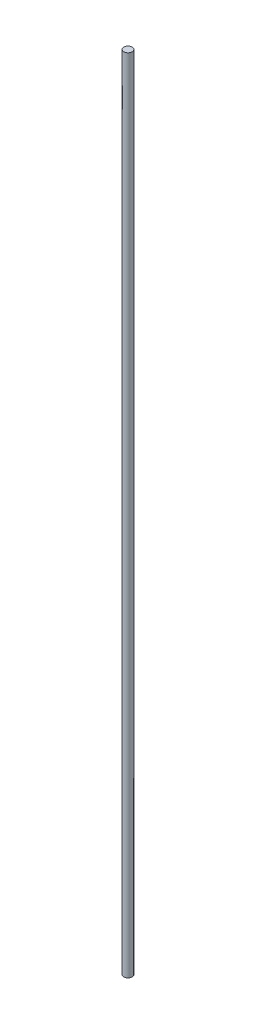
from build123d import *

# Parameters (mm, degrees)
SKETCH1_W = 0.25
SKETCH1_H = 48


with BuildPart() as part:
    # Sketch1 → Revolve1 (revolve)
    with BuildSketch(Plane.XY, mode=Mode.PRIVATE) as revolve1_sk:
        with Locations((-0.125, 24)):
            Rectangle(SKETCH1_W, SKETCH1_H)
    revolve(revolve1_sk.sketch.rotate(Axis((0, 0, 0), (0, 1, 0)), 270), axis=Axis((0, 0, 0), (0, 1, 0)))


solid = part.part
